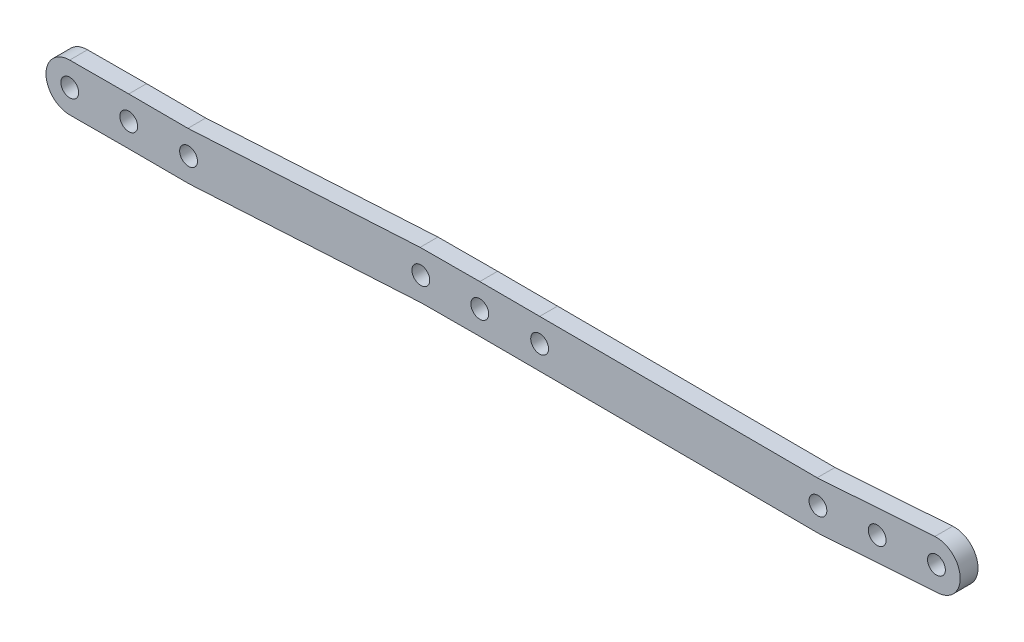
SolidWorks part; units mm, degrees
ref_plane "Front Plane" through (0, 0, 0) normal (0, 0, 1) x (1, 0, 0)
ref_plane "Top Plane" through (0, 0, 0) normal (0, 1, 0) x (1, 0, 0)
ref_plane "Right Plane" through (0, 0, 0) normal (1, 0, 0) x (0, 0, -1)
other "Configuration Table"
sketch "Sketch1" plane through (0, 0, 0) normal (0, 0, 1) x (1, 0, 0)
  line L0 (-69.0324, -2.2273) -> (-59.102, -2.1963) construction
  line L1 (-59.102, -2.1963) -> (-49.0324, -2.2273) construction
  line L2 (-49.0324, -2.2273) -> (-9.9259, -0.0331) construction
  line L3 (-9.9259, -0.0331) -> (0, 0) construction
  line L4 (0, 0) -> (10.0741, -0.0331) construction
  line L5 (10.0741, -0.0331) -> (56.9321, -0.2061) construction
  line L6 (56.9321, -0.2061) -> (66.9092, 0.4705) construction
  line L7 (66.9092, 0.4705) -> (76.8863, 1.147) construction
  line L8 (-69.0199, -6.2273) -> (-59.1019, -6.1963)
  line L9 (-59.1019, -6.1963) -> (-48.9265, -6.2277)
  line L10 (-48.9265, -6.2277) -> (-9.8071, -4.0327)
  line L11 (-9.8071, -4.0327) -> (0.0001, -4)
  line L12 (0.0001, -4) -> (10.0602, -4.0331)
  line L13 (10.0602, -4.0331) -> (57.0602, -4.2066)
  line L14 (57.0602, -4.2066) -> (67.1798, -3.5204)
  line L15 (67.1798, -3.5204) -> (77.1569, -2.8438)
  line L16 (-69.0449, 1.7726) -> (-59.1021, 1.8037)
  line L17 (-59.1021, 1.8037) -> (-49.1384, 1.773)
  line L18 (-49.1384, 1.773) -> (-10.0446, 3.9665)
  line L19 (-10.0446, 3.9665) -> (-0.0001, 4)
  line L20 (-0.0001, 4) -> (10.0881, 3.9669)
  line L21 (10.0881, 3.9669) -> (56.804, 3.7944)
  line L22 (56.804, 3.7944) -> (66.6386, 4.4613)
  line L23 (66.6386, 4.4613) -> (76.6157, 5.1378)
  circle A0 centre (-69.0324, -2.2273) radius 1.5
  circle A1 centre (-59.102, -2.1963) radius 1.5
  circle A2 centre (-49.0324, -2.2273) radius 1.5
  circle A3 centre (-9.9259, -0.0331) radius 1.5
  circle A4 centre (0, 0) radius 1.5
  circle A5 centre (10.0741, -0.0331) radius 1.5
  circle A6 centre (56.9321, -0.2061) radius 1.5
  circle A7 centre (66.9092, 0.4705) radius 1.5
  circle A8 centre (76.8863, 1.147) radius 1.5
  arc A9 (-69.0449, 1.7726) -> (-69.0199, -6.2273) centre (-69.0324, -2.2273) ccw
  arc A10 (77.1569, -2.8438) -> (76.6157, 5.1378) centre (76.8863, 1.147) ccw
  dimension "D1" = 3
  dimension "D4" = 4
extrude "Boss-Extrude1" add sketch "Sketch1" along normal blind 3
